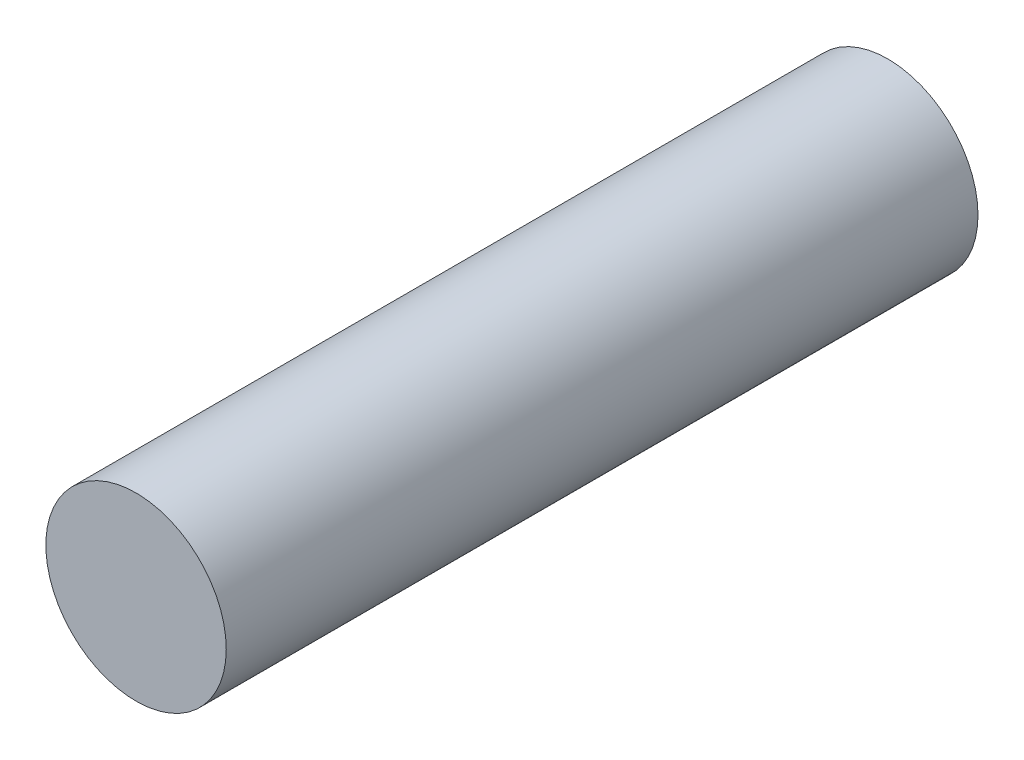
SolidWorks part; units mm, degrees
ref_plane "Front Plane" through (0, 0, 0) normal (0, 0, 1) x (1, 0, 0)
ref_plane "Top Plane" through (0, 0, 0) normal (0, 1, 0) x (1, 0, 0)
ref_plane "Right Plane" through (0, 0, 0) normal (1, 0, 0) x (0, 0, -1)
other "Configuration Table"
sketch "Sketch1" plane through (0, 0, 0) normal (0, 0, 1) x (1, 0, 0)
  circle A0 centre (0, 0) radius 12
  dimension "D1" = 24
extrude "Boss-Extrude1" add sketch "Sketch1" along normal blind 100
